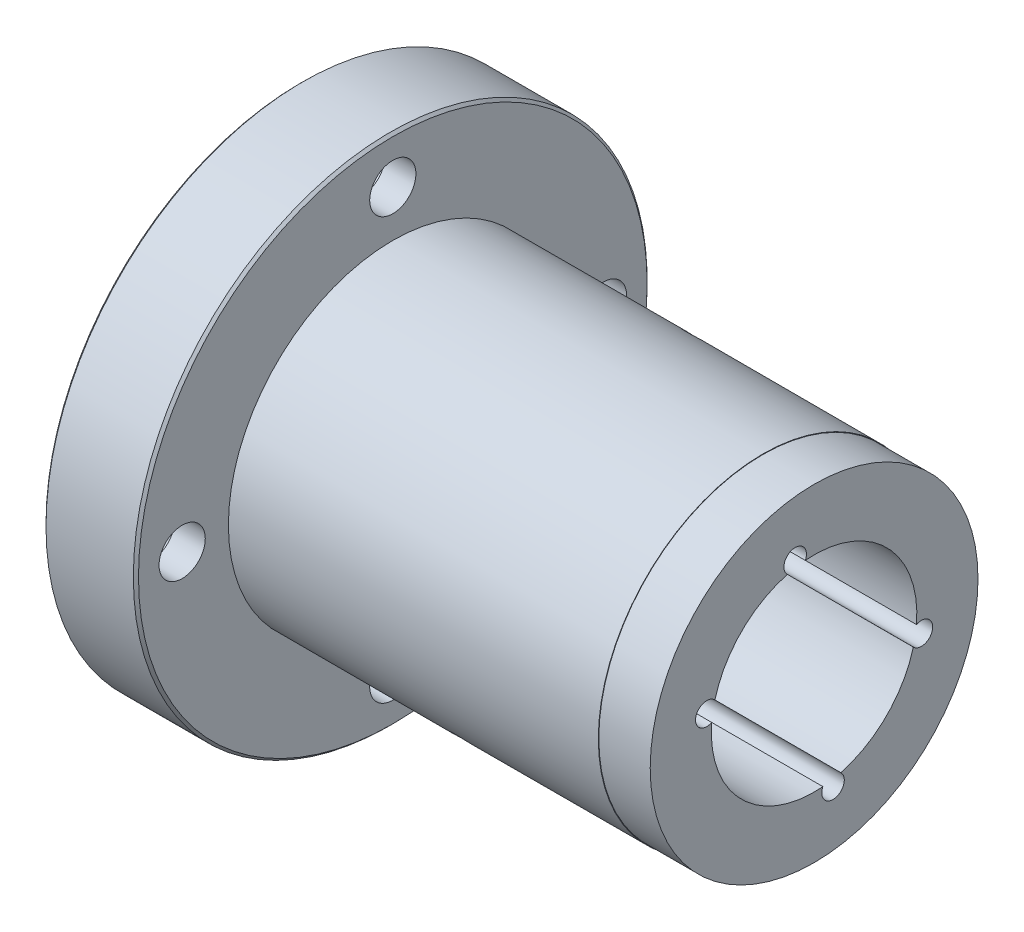
from build123d import *

# Parameters (mm, degrees)
CUT_EXTRUDE_1_DEPTH      = 50
CUT_EXTRUDE_1_DEPTH_BACK = 50
CUT_EXTRUDE_2_DEPTH      = 50
CUT_EXTRUDE_2_DEPTH_BACK = 50
SKETCH_13_W              = 10
SKETCH_13_H              = 31.9


with BuildPart() as part:
    # 草图1 → 旋转1 (revolve)
    with BuildSketch(Plane.XY, mode=Mode.PRIVATE) as revolve_1_sk:
        Polygon((-50, 49.5), (-50, 20), (50, 20), (50, 31.9), (40, 31.9), (40, 32), (-32, 32), (-32, 49.5), (-32.5, 50), (-49.5, 50), align=None)
    revolve(revolve_1_sk.sketch.rotate(Axis((50, 0, 0), (-1, 0, 0)), 270), axis=Axis((50, 0, 0), (-1, 0, 0)))

    # 草图2 → 切除-拉伸1 (cut, two sides: drawn at the far end of the back side and taken through both)
    with BuildSketch(Plane(origin=(0, 0, 0), x_dir=(0, 0, -1), z_dir=(1, 0, 0)).offset(-CUT_EXTRUDE_1_DEPTH_BACK)):
        with BuildLine():
            ThreePointArc((-5.203224708, 19.311303753), (-19.69615506, -3.472963553), (1.715423015, -19.926297295))
            ThreePointArc((1.715423015, -19.926297295), (4.063367357, -23.04450142), (5.203224708, -19.311303753))
            ThreePointArc((5.203224708, -19.311303753), (19.69615506, 3.472963553), (-1.715423015, 19.926297295))
            ThreePointArc((-1.715423015, 19.926297295), (-4.063367357, 23.04450142), (-5.203224708, 19.311303753))
        make_face()
    extrude(amount=CUT_EXTRUDE_1_DEPTH + CUT_EXTRUDE_1_DEPTH_BACK, mode=Mode.SUBTRACT)

    # 草图3 → 切除-拉伸2 (cut, two sides: drawn at the far end of the back side and taken through both)
    with BuildSketch(Plane(origin=(0, 0, 0), x_dir=(0, 0, -1), z_dir=(1, 0, 0)).offset(-CUT_EXTRUDE_2_DEPTH_BACK)):
        with BuildLine():
            ThreePointArc((-19.311303753, 5.203224708), (-23.04450142, 4.063367357), (-19.926297295, 1.715423015))
            ThreePointArc((-19.926297295, 1.715423015), (-3.472963553, -19.69615506), (19.311303753, -5.203224708))
            ThreePointArc((19.311303753, -5.203224708), (23.04450142, -4.063367357), (19.926297295, -1.715423015))
            ThreePointArc((19.926297295, -1.715423015), (3.472963553, 19.69615506), (-19.311303753, 5.203224708))
        make_face()
    extrude(amount=CUT_EXTRUDE_2_DEPTH + CUT_EXTRUDE_2_DEPTH_BACK, mode=Mode.SUBTRACT)

    # 草图4 → 切除-旋转1 (revolve, cut)
    with BuildSketch(Plane(origin=(4, 0, 0), x_dir=(0, 0, -1), z_dir=(1, 0, 0)), mode=Mode.PRIVATE) as cut_revolve_1_sk:
        Polygon((-23.334523779, -23.334523779), (-24.748737342, -21.920310217), (21.920310217, 24.748737342), (23.334523779, 23.334523779), align=None)
    revolve(cut_revolve_1_sk.sketch.rotate(Axis((4, 23.334523779, -23.334523779), (0, -0.7071067811865476, 0.7071067811865476)), 180), axis=Axis((4, 23.334523779, -23.334523779), (0, -0.7071067811865476, 0.7071067811865476)), mode=Mode.SUBTRACT)

    # 草图5 → 旋转2 (revolve)
    with BuildSketch(Plane(origin=(0, 0, 0), x_dir=(1, 0, 0), z_dir=(0, -0.17364817766693041, 0.9848077530122081)), mode=Mode.PRIVATE) as revolve_2_sk:
        with BuildLine():
            Line((-10.948, -21.211), (10.948, -21.211))
            ThreePointArc((10.948, -21.211), (8.781398718, -23.400874996), (6.5685, -21.257794765))
            ThreePointArc((6.5685, -21.257794765), (4.379, -23.401), (2.1895, -21.257794765))
            ThreePointArc((2.1895, -21.257794765), (0, -23.401), (-2.1895, -21.257794765))
            ThreePointArc((-2.1895, -21.257794765), (-4.379, -23.401), (-6.5685, -21.257794765))
            ThreePointArc((-6.5685, -21.257794765), (-8.781398718, -23.400874996), (-10.948, -21.211))
        make_face()
    revolve(revolve_2_sk.sketch.rotate(Axis((-10.948, -20.888757249, -3.683251496), (1, 0, 0)), 80), axis=Axis((-10.948, -20.888757249, -3.683251496), (1, 0, 0)))

    # 草图6 → 旋转3 (revolve)
    with BuildSketch(Plane(origin=(0, 0, 0), x_dir=(1, 0, 0), z_dir=(0, -0.17364817766693041, 0.9848077530122081)), mode=Mode.PRIVATE) as revolve_3_sk:
        with BuildLine():
            Line((10.948, 21.211), (-10.948, 21.211))
            ThreePointArc((-10.948, 21.211), (-8.781398718, 23.400874996), (-6.5685, 21.257794765))
            ThreePointArc((-6.5685, 21.257794765), (-4.379, 23.401), (-2.1895, 21.257794765))
            ThreePointArc((-2.1895, 21.257794765), (0, 23.401), (2.1895, 21.257794765))
            ThreePointArc((2.1895, 21.257794765), (4.379, 23.401), (6.5685, 21.257794765))
            ThreePointArc((6.5685, 21.257794765), (8.781398718, 23.400874996), (10.948, 21.211))
        make_face()
    revolve(revolve_3_sk.sketch.rotate(Axis((10.948, 20.888757249, 3.683251496), (-1, 0, 0)), 280), axis=Axis((10.948, 20.888757249, 3.683251496), (-1, 0, 0)))

    # 草图7 → 旋转4 (revolve)
    with BuildSketch(Plane(origin=(0, 0, 0), x_dir=(-1, 0, 0), z_dir=(0, -0.9848077530122081, 0.17364817766693047)), mode=Mode.PRIVATE) as revolve_4_sk:
        with BuildLine():
            Line((10.948, 21.211), (-10.948, 21.211))
            ThreePointArc((-10.948, 21.211), (-8.781398718, 23.400874996), (-6.5685, 21.257794765))
            ThreePointArc((-6.5685, 21.257794765), (-4.379, 23.401), (-2.1895, 21.257794765))
            ThreePointArc((-2.1895, 21.257794765), (0, 23.401), (2.1895, 21.257794765))
            ThreePointArc((2.1895, 21.257794765), (4.379, 23.401), (6.5685, 21.257794765))
            ThreePointArc((6.5685, 21.257794765), (8.781398718, 23.400874996), (10.948, 21.211))
        make_face()
    revolve(revolve_4_sk.sketch.rotate(Axis((-10.948, -3.683251496, -20.888757249), (1, 0, 0)), 10), axis=Axis((-10.948, -3.683251496, -20.888757249), (1, 0, 0)))

    # 草图8 → 旋转5 (revolve)
    with BuildSketch(Plane(origin=(0, 0, 0), x_dir=(-1, 0, 0), z_dir=(0, -0.9848077530122081, 0.17364817766693047)), mode=Mode.PRIVATE) as revolve_5_sk:
        with BuildLine():
            Line((-10.948, -21.211), (10.948, -21.211))
            ThreePointArc((10.948, -21.211), (8.781398718, -23.400874996), (6.5685, -21.257794765))
            ThreePointArc((6.5685, -21.257794765), (4.379, -23.401), (2.1895, -21.257794765))
            ThreePointArc((2.1895, -21.257794765), (0, -23.401), (-2.1895, -21.257794765))
            ThreePointArc((-2.1895, -21.257794765), (-4.379, -23.401), (-6.5685, -21.257794765))
            ThreePointArc((-6.5685, -21.257794765), (-8.781398718, -23.400874996), (-10.948, -21.211))
        make_face()
    revolve(revolve_5_sk.sketch.rotate(Axis((10.948, 3.683251496, 20.888757249), (-1, 0, 0)), 350), axis=Axis((10.948, 3.683251496, 20.888757249), (-1, 0, 0)))

    # 草图9 → 切除-旋转2 (revolve, cut)
    with BuildSketch(Plane.XY, mode=Mode.PRIVATE) as cut_revolve_2_sk:
        Polygon((-50, 41), (-50, 48), (-38, 48), (-38, 45.5), (-32, 45.5), (-32, 41), align=None)
    revolve(cut_revolve_2_sk.sketch.rotate(Axis((-32, 41, 0), (-1, 0, 0)), 270), axis=Axis((-32, 41, 0), (-1, 0, 0)), mode=Mode.SUBTRACT)

    # 草图10 → 切除-旋转3 (revolve, cut)
    with BuildSketch(Plane.XY, mode=Mode.PRIVATE) as cut_revolve_3_sk:
        Polygon((-32, -41), (-32, -45.5), (-38, -45.5), (-38, -48), (-50, -48), (-50, -41), align=None)
    revolve(cut_revolve_3_sk.sketch.rotate(Axis((-50, -41, 0), (1, 0, 0)), 90), axis=Axis((-50, -41, 0), (1, 0, 0)), mode=Mode.SUBTRACT)

    # 草图11 → 切除-旋转4 (revolve, cut)
    with BuildSketch(Plane(origin=(0, 0, 0), x_dir=(1, 0, 0), z_dir=(0, 1, 0)), mode=Mode.PRIVATE) as cut_revolve_4_sk:
        Polygon((-50, 41), (-50, 48), (-38, 48), (-38, 45.5), (-32, 45.5), (-32, 41), align=None)
    revolve(cut_revolve_4_sk.sketch.rotate(Axis((-32, 0, -41), (-1, 0, 0)), 180), axis=Axis((-32, 0, -41), (-1, 0, 0)), mode=Mode.SUBTRACT)

    # 草图12 → 切除-旋转5 (revolve, cut)
    with BuildSketch(Plane(origin=(0, 0, 0), x_dir=(1, 0, 0), z_dir=(0, 1, 0)), mode=Mode.PRIVATE) as cut_revolve_5_sk:
        Polygon((-32, -41), (-32, -45.5), (-38, -45.5), (-38, -48), (-50, -48), (-50, -41), align=None)
    revolve(cut_revolve_5_sk.sketch.rotate(Axis((-50, 0, 41), (1, 0, 0)), 180), axis=Axis((-50, 0, 41), (1, 0, 0)), mode=Mode.SUBTRACT)

    # 草图13 → 切除-旋转6 (revolve, cut)
    with BuildSketch(Plane.XY, mode=Mode.PRIVATE) as cut_revolve_6_sk:
        with Locations((-45, 15.95)):
            Rectangle(SKETCH_13_W, SKETCH_13_H)
    revolve(cut_revolve_6_sk.sketch.rotate(Axis((-40, 0, 0), (-1, 0, 0)), 180), axis=Axis((-40, 0, 0), (-1, 0, 0)), mode=Mode.SUBTRACT)


solid = part.part
